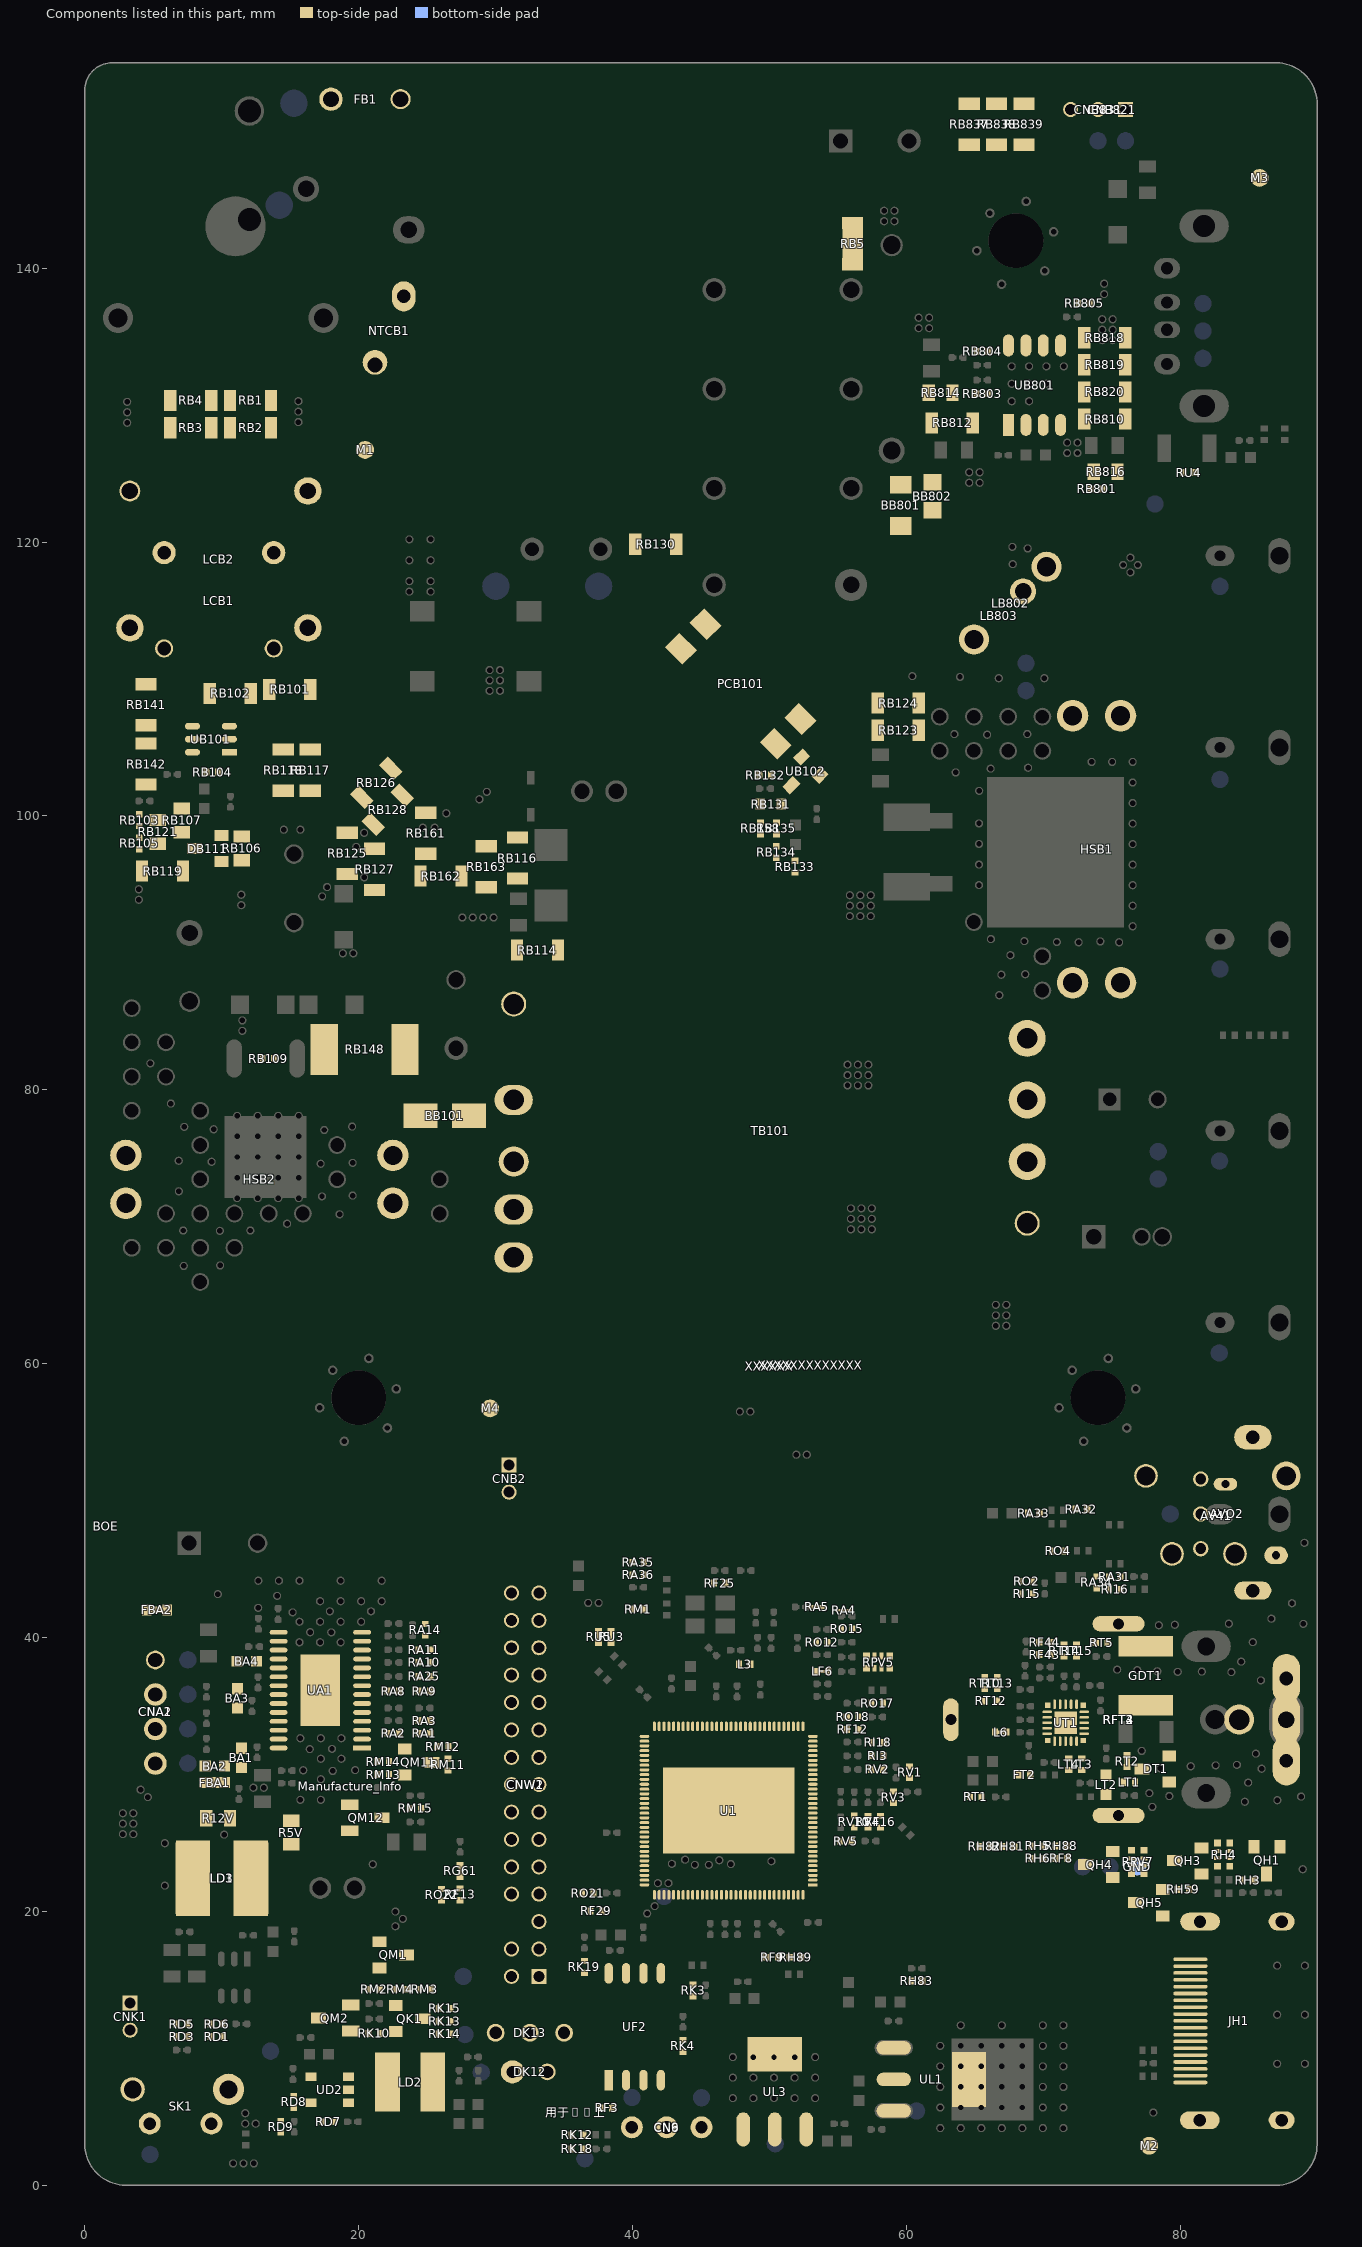
[diagram p0: the components of this part, seen from the top]
# Altium PCB MISC116569.PcbDoc (part 4 of 15)
Units mm, origin at the board's own origin, x right, y up, seen from the top; angles counter-clockwise.
Board outline 90 x 155 mm, 2 copper layers (TopLayer, BottomLayer), stack 1.571 mm thick; 527 components, 277 nets, 2450 pads, 649 vias.

## Footprints (in the part's own frame and the unit in brackets; to place one, negate y for a bottom-side part, rotate by r counter-clockwise, add the part's x,y. Pads: shape width x height; smd on the part's side, far side on the other; paste and mask are expansions set on the pad) (continued)
"FUSE8.5*4-V-5(T3.15AL 250V~)" [mm] "SMT1315AP/2010T1A250VA1(编带/华德)"
  round 1.7 hole 1.15: 1(2.54,0)
  round 1.473 / inner round 1.7 / far side round 1.7 hole 1.15: 2(-2.54,0)
  round 1.9 on Top Overlay: 4(2.54,0) 5(-2.54,0)
  BottomLayer lines w1: 2.54,0 2.562,-0.022 3.977,-1.437 ; 2.312,-0.271 2.338,-0.289 2.367,-0.31 3.499,-1.103 3.977,-1.437 ; -2.312,0.271 -2.338,0.289 -2.376,0.316 -2.933,0.706 -3.977,1.437 ; -2.54,0 -3.011,0.471 -3.977,1.437 ; -2.811,-0.228 -2.829,-0.202 ; 3.977,-1.437 2.971,0 2.844,0.182 ; 2.844,0.182 2.844,0.182 ; 2.844,0.182 2.829,0.202 2.812,0.227 ; 2.812,0.227 2.811,0.228 ; -2.829,-0.202 -2.839,-0.189 -2.973,0.003 -3.096,0.179 -3.165,0.277 -3.828,1.224 -3.977,1.437 ; -2.829,-0.202 -2.829,-0.202 ; -2.829,-0.202 -2.829,-0.202 ; -3.977,1.437 -3.977,1.437
  silkscreen extent -4.3,-2.1 4.3,2.1, body extent -4.3,-2.1 4.3,2.1, height 8.5
GND#1 [mm] "导通线"
  rect 0.66x0.178 smd paste-0.45 mask-0.45: JP_1K(-0.32,0) JP_2K(0.32,0)
GND#2 [mm] "导通线"
  rect 0.66x0.3 smd paste-0.45 mask-0.45: JP_1K(-0.32,0) JP_2K(0.32,0)
HDMI-HS-1 [mm] "浙江和丰   HHF-14B000-2SA。17.09.25更新钢网;171107更新焊盘露铜位置;18.04.19 更新大脚孔径;19.09.11 更新端子视图开口高度(6.1-6.2,0."
  rect 2.2x3.8 on Top Paste: 0(-7.75,4.18) 0(7.753,4.183)
  rect 2.2x6 on Top Paste: 0(-7.75,9.355) 0(7.75,9.355)
  oval 0.26x2.5 smd: 1(4.5,11.258) 2(4,11.258) 3(3.5,11.258) 4(3,11.258) 5(2.5,11.258) 6(2,11.258) 7(1.5,11.258) 8(1,11.258) 9(0.5,11.258) 10(0,11.258) 11(-0.5,11.258) 12(-1,11.258) 13(-1.5,11.258) 14(-2,11.258) 15(-2.5,11.258) 16(-3,11.258) 17(-3.5,11.258) 18(-4,11.258) 19(-4.5,11.258)
  oval 1.3x2.9 hole 0.9 slot 2.5 at 90 deg mask+0.076: 20(-7.25,10.565) 22(7.25,10.55)
  oval 1.3x1.9 hole 0.9 slot 1.5 at 90 deg mask+0.076: 21(-7.25,4.59) 23(7.25,4.59)
  silkscreen extent -7.5,2 7.5,12.19, body extent -10.25,-57.68 10.25,12.17, height 8.92
"Heat-Shrinkable Tube" [mm] "收缩前壁厚0.3+-0.05，收缩后壁厚0.6+-0.1"
  round 0.3 on Mech2: 0(0,0)
"High Voltage" [mm]
  silkscreen extent -0.53,-1.52 0.43,1.27
HOT [mm]
HS151-TEMP-NG [mm] "散热片.临时封装.10/21/2019"
  oval 1.9x2.4 on Top Overlay: 0(-9.75,-1.75) 0(-9.75,1.75) 0(9.75,-1.75) 0(9.75,1.75)
  round 3 on Bottom Solder: 0(-9.75,-1.75) 0(-9.75,1.75) 0(9.75,-1.75) 0(9.75,1.75)
  round 2.3 hole 1.4: 1(-9.75,1.75) 2(-9.75,-1.75) 3(9.75,-1.75) 4(9.75,1.75)
  silkscreen extent -10.03,-2.93 10.03,2.93
HS(15X15X5)-S [mm] "YT.YT-P-151505.2019/9/18"
  silkscreen extent -7.63,-7.63 7.63,7.63, body extent -7.5,-7.5 7.5,7.5, height 5
KEY-HD-6 [mm] "春生KFC-A06--E-4-160-7.5/4; 中心高度为4mm;14.09.04;171102修正突出距离"
  round 2.5 on Top Overlay: 0(-3.5,5) 0(3.5,5)
  round 1.8 on Top Overlay: 0(-2.25,2.5) 0(2.25,2.5)
  round 1.6 hole 0.9: 1(2.25,2.5) 2(-2.25,2.5)
  round 2.286 hole 1.3: 3(3.5,5)
  round 1.778 / inner round 2.286 / far side round 2.286 hole 1.3: 4(-3.5,5)
  silkscreen extent -3.85,0 3.85,6.6
L0402 [mm] "电感"
  rect 0.45x0.55 smd mask+0.076: 1(-0.425,0) 2(0.425,0)
  silkscreen extent -0.8,-0.42 0.8,0.43, body extent -0.5,-0.25 0.5,0.25, height 0.5
L0603 [mm] "片式磁珠、电感、ESD"
  rect 0.813x0.8 smd mask+0.076: 1(-0.706,0) 2(0.706,0)
  silkscreen extent -1.27,-0.55 1.27,0.55, body extent -0.8,-0.4 0.8,0.4, height 0.8
L0805 [mm] "片式磁珠、电感"
  rect 1.2x1.3 smd: 1(-1.016,0) 2(1.016,0)
  silkscreen extent -1.92,-0.95 1.92,0.95, body extent -1,-0.62 1,0.63, height 1.25
L1206 [mm] "磁珠"
  rect 1.3x1.6 smd: 1(-1.5,-0.001) 2(1.5,0.001)
  silkscreen extent -2.55,-1.2 2.55,1.2, body extent -1.6,-0.8 1.6,0.8, height 1.25
L(4*3*2.55)-S [mm] "贴片磁珠；SMB -302540-K5B- L1;15.02.05（17.12.07更新高度信息）"
  rect 2.5x1.8 smd: 1(-1.775,0) 2(1.775,0)
  silkscreen extent -2.12,-1.6 2.12,1.6, body extent -2.55,-1.6 2.55,1.6, height 2.7
L(4.5*3.5)-S [mm] "SMD4532-6R8M-023"
  rect 1.8x4.3 smd: 1(-1.65,0) 2(1.65,0)
  TopLayer pour cut-out: -0.76,2.15 0.796,2.15 0.796,2.141 0.796,-2.149 -0.756,-2.149 -0.756,-2.15
  silkscreen extent -2.83,-2.44 3.3,2.44
L(5.8*4.5)-S [mm] "APC52A45M4R7\电感\Cailank;170317更新阻焊兼容L(4*3.0)-S"
  rect 2.5x5.5 smd paste-5.5: 1(2.105,0) 2(-2.105,0)
  TopLayer pour cut-out: -0.849,2.746 -0.845,2.75 0.861,2.75 0.861,-2.749 0.861,-2.753 0.859,-2.753 -0.862,-2.753
  silkscreen extent -1.5,-2.9 3.88,2.9, body extent -3.06,-2.65 3.08,2.74, height 4.8
L(6.0*4.5)-S [mm] "SWPA6045S4R7MT(Sunlord) :功率电感;161103更新焊盘大小"
  rect 2.1x5.2 smd paste-6: 1(-2.35,0) 2(2.35,0)
  TopLayer pour cut-out: -1.282,2.552 1.294,2.543 1.297,-2.547 -1.311,-2.549
  silkscreen extent -3.16,-3.15 3.9,3.15, body extent -3,-3 3,3, height 4.5
L(13.5*15.5)-V-5 [mm] "深圳秀益达；SA-A048-036-A SPK1214RBL-680K；14.11.19"
  round 1.9 hole 1.2 mask+0.076: 1(-2.5,0) 2(2.5,0)
  round 2.1 on Top Overlay mask+0.076: 3(-2.5,0) 4(2.5,0)
  silkscreen extent -6.75,-6.75 6.75,6.75, body extent -9.53,-9.51 9.52,9.53, height 15.5
L/LC2/15*14.5-V7.5 [mm] "SYDR1212-L003-YMX"
  round 2.2 hole 1.4: 1(-3.75,0) 2(3.75,0)
  round 2.4 on Top Overlay: 1(-3.75,0) 1(3.75,0)
  silkscreen extent -7.25,-7.25 7.25,7.25
L/LC4/UU9.8/7*8-H [mm] "汉(玛电子UU9.8-26mH)"
  round 1.7 hole 1: 1(-4,-3.5) 2(4,-3.5)
  round 1.321 / inner round 1.7 / far side round 1.7 hole 1: 3(4,3.5) 4(-4,3.5)
  round 1.9 on Top Overlay: 17(-4,3.5) 18(4,3.5) 19(4,-3.5) 20(-4,-3.5)
  silkscreen extent -8.5,-11 8.5,5
L/UU10.5/10*13-2 [mm] "SYUU10.5-L001(协兴电子) 卡扣在侧面"
  round 2 hole 1.2: 1(5,-6.5) 3(-5,6.5) 4(-5,-6.5)
  round 1.524 / inner round 2 / far side round 2 hole 1.2: 2(5,6.5)
  round 2.2 on Top Overlay: 4(-5,6.5) 4(-5,-6.5) 4(5,6.5) 4(5,-6.5)
  silkscreen extent -8,-9.25 11.5,9.25, body extent -8,-8.5 9.5,8.5, height 13.8
LED-HD-5 [mm] "HZFT503094CPBR-1(红、蓝);14.06.27"
  oval 1.5x1.7 on Top Overlay: 0(-2.502,0.002) 0(-0.002,0.002) 0(2.498,0.002)
  round 1.3 / inner oval 1.3x1.5 / far side oval 1.5x2 hole 0.9: 1(-2.502,0.002) 2(-0.002,0.002) 3(2.498,0.002)
  silkscreen extent -2.81,-11.06 2.8,2.6
LED-HD-6 [mm] "厦门华联；HFR803099P(P5D2)-S5(SN)；14.09.03"
  round 1.9 on Top Overlay mask+0.076: 3(1.27,2.65) 4(-1.27,2.65)
  round 1.7 hole 0.9 mask+0.076: A(-1.27,2.65)
  round 1.219 / inner round 1.7 / far side round 1.7 hole 0.9 mask+0.076: K(1.27,2.65)
  silkscreen extent -2.02,-5.62 2.02,4.02
MANUFACTURE_INFO [mm]
  round 0.3 on Mech2: 0(0,0)
MARK [mm] "SMD 使用"
  round 1.3 smd paste+0 mask+0.65: 0(0,0)
  TopLayer circle w0.254: c0,0 r1.444
  TopLayer pour cut-out: -1.3,0 -1.201,-0.497 -0.919,-0.919 -0.497,-1.201 0,-1.3 0,-1.3 0.497,-1.201 0.919,-0.919 1.201,-0.497 1.3,0 1.3,0 1.201,0.497 0.919,0.919 0.497,1.201 0,1.3 0,1.3 -0.497,1.201 -0.919,0.919 -1.201,0.497 -1.3,0
Mylar [mm] "180×180×0.4mm-PC-黑色"
NTC(10*5)-V5 [mm] "热敏电阻 SCK152R58MSY  (为勤电子）;161022更新椭圆孔"
  round 1.8 hole 1.1 copper offset 0.178,0: 1(-2.5,1.05)
  round 2 on Top Overlay: 2(-2.5,1.05)
  oval 2.2x1.7 hole 1 slot 1.5 at 0 deg: 2(2.5,-1.05)
  oval 2.4x1.9 on Top Overlay: 3(2.5,-1.05)
  silkscreen extent -5.77,-2.5 5.77,2.5, body extent -5.75,-2 5.75,2, height 13.75
OC4-S-1 [mm] "巨路国际；肖特基LTV-817S-TA-B"
  rect 1.5x1.8 smd: 1(-1.27,-4.9) 2(1.27,-4.9) 3(1.27,4.9) 4(-1.27,4.9)
  silkscreen extent -3.17,-5.35 2.55,3.5, body extent -6.95,-6.95 6.95,6.95, height 3.88
OPTICAL-HD-3 [mm] "强生GQ-03-08  通用封装 (TR）  塑胶整体高度11.6mm，中心高度6mm(17.04.28,增加丝印宽度到12.3mm）"
  oval 2x3.4 on Top Overlay: 0(-5.6,4.7) 0(5.6,4.7)
  round 1.778 on Top Overlay: 0(-2.54,8.5) 0(0,8.5) 0(2.54,8.5)
  round 1.118 / inner round 1.524 / far side round 1.524 hole 0.8: 1(-2.54,8.5) 2(0,8.5) 3(2.54,8.5)
  oval 1.321x2.718 / inner oval 1.8x3.2 / far side oval 1.8x3.2 hole 1 slot 2.4 at 90 deg: 4(-5.6,4.7)
  oval 1.8x2.718 / inner oval 1.8x3.2 / far side oval 1.8x3.2 hole 1 slot 2.4 at 90 deg: 5(5.6,4.7)
  silkscreen extent -6.15,0 6.15,11.8
PCB_NAME [mm]
  round 0.3 on Mech2: 0(0,0)
PCB_TIME [mm]
  round 0.3 on Mech2: 0(0,0)
PHONE-HD-42 [mm] "YUQIU;PJ7724-F05L3BE-D;160401(17.07.18,孔内边增加0.1mm，外距不变）(18.03.13 更新孔径）"
  oval 1.5x2.3 on Top Overlay: 0(-3,3) 8(2.2,6.7)
  round 2.3 on Top Overlay: 0(-2.9,10.6) 0(-2.9,6) 0(2.8,12.5) 0(2.8,2.25)
  round 2.1 hole 1.4: 1(2.8,2.25)
  oval 1.3x1.727 / inner oval 1.3x2.1 / far side oval 1.3x2.1 hole 0.6 slot 1.4 at 90 deg: 2(-3,3)
  round 1.727 / inner round 2.1 / far side round 2.1 hole 1.4: 3(2.8,12.5) 4(-2.9,6) 5(-2.9,10.6)
  oval 0.914x1.727 / inner oval 1.3x2.1 / far side oval 1.3x2.1 hole 0.6 slot 1.4 at 90 deg: 6(2.2,6.7)
  silkscreen extent -3.65,0 3.65,13.15, body extent -5.05,-62.22 5.05,13, height 12.05
QFN24/0.4-1 [mm] "Si2151;14-03-17;161116新增两个EPAD孔"
  rect 0.4x0.4 smd: 1(-1.295,1.295) 7(-1.295,-1.295) 13(1.295,-1.295) 19(1.295,1.295)
  oval 0.7x0.2 smd: 2(-1.35,0.8) 3(-1.35,0.4) 4(-1.35,0) 6(-1.35,-0.8) 14(1.35,-0.8) 15(1.35,-0.4) 16(1.35,0) 17(1.35,0.4) 18(1.35,0.8)
  oval 0.7x0.2 smd paste+0: 5(-1.35,-0.4)
  oval 0.2x0.7 smd: 8(-0.8,-1.35) 9(-0.4,-1.35) 10(0,-1.35) 11(0.4,-1.35) 12(0.8,-1.35) 20(0.8,1.35) 21(0.4,1.35) 22(0,1.35) 23(-0.4,1.35)
  oval 0.2x0.7 smd paste+0: 24(-0.8,1.35)
  rect 1.651x1.651 smd paste-2 mask-2: EPAD(0,0)
  silkscreen extent -2.6,-2.24 2.11,2.24, body extent -1.5,-1.5 1.5,1.5, height 0.9
QFN128/0.35-1 [mm] "Mstar,TSUMV53RWUT-Z1,18.11.16(19.03.30   减少外延焊盘长度）(19.04.23 更新钢网尺寸）（因温升修改为12宫格）"
  oct 2.2x1.9 on Top Paste: 0(-3.7,0) 0(-3.697,-2.145) 0(-3.697,2.145) 0(-1.253,2.145) 0(-1.253,-2.145) 0(-1.25,0) 0(1.247,2.145) 0(1.247,-2.145) 0(1.25,0) 0(3.697,-2.145) 0(3.697,2.145) 0(3.7,0)
  oct 2.2x1.9 on Top Solder: 0(-3.7,0) 0(-3.697,-2.145) 0(-3.697,2.145) 0(-1.253,2.145) 0(-1.253,-2.145) 0(-1.25,0) 0(1.247,2.145) 0(1.247,-2.145) 0(1.25,0) 0(3.697,-2.145) 0(3.697,2.145) 0(3.7,0)
  rect 0.7x0.22 smd paste-0.02 mask-0.035: 1(-6.151,5.425)
  oval 0.7x0.22 smd paste-0.02 mask-0.035: 2(-6.151,5.075) 3(-6.151,4.725) 4(-6.151,4.375) 5(-6.151,4.025) 6(-6.151,3.675) 7(-6.151,3.325) 8(-6.151,2.975) 9(-6.151,2.625) 10(-6.151,2.275) 11(-6.151,1.925) 12(-6.151,1.575) 13(-6.151,1.225) 14(-6.151,0.875) 15(-6.151,0.525) 16(-6.151,0.175) 17(-6.151,-0.175) 18(-6.151,-0.525) 19(-6.151,-0.875) 20(-6.151,-1.225) 21(-6.151,-1.575) 22(-6.151,-1.925) 23(-6.151,-2.275) 24(-6.151,-2.625) 25(-6.151,-2.975) 26(-6.151,-3.325) 27(-6.151,-3.675) 28(-6.151,-4.025) 29(-6.151,-4.375) 30(-6.151,-4.725) 31(-6.151,-5.075) 32(-6.151,-5.425) 65(6.151,-5.425) 66(6.151,-5.075) 67(6.151,-4.725) 68(6.151,-4.375) 69(6.151,-4.025) 70(6.151,-3.675) 71(6.151,-3.325) 72(6.151,-2.975) 73(6.151,-2.625) 74(6.151,-2.275) 75(6.151,-1.925) 76(6.151,-1.575) 77(6.151,-1.225) 78(6.151,-0.875) 79(6.151,-0.525) 80(6.151,-0.175) 81(6.151,0.175) 82(6.151,0.525) 83(6.151,0.875) 84(6.151,1.225) 85(6.151,1.575) 86(6.151,1.925) 87(6.151,2.275) 88(6.151,2.625) 89(6.151,2.975) 90(6.151,3.325) 91(6.151,3.675) 92(6.151,4.025) 93(6.151,4.375) 94(6.151,4.725) 95(6.151,5.075) 96(6.151,5.425)
  oval 0.22x0.7 smd paste-0.02 mask-0.035: 33(-5.425,-6.151) 34(-5.075,-6.151) 35(-4.725,-6.151) 36(-4.375,-6.151) 37(-4.025,-6.151) 38(-3.675,-6.151) 39(-3.325,-6.151) 40(-2.975,-6.151) 41(-2.625,-6.151) 42(-2.275,-6.151) 43(-1.925,-6.151) 44(-1.575,-6.151) 45(-1.225,-6.151) 46(-0.875,-6.151) 47(-0.525,-6.151) 48(-0.175,-6.151) 49(0.175,-6.151) 50(0.525,-6.151) 51(0.875,-6.151) 52(1.225,-6.151) 53(1.575,-6.151) 54(1.925,-6.151) 55(2.275,-6.151) 56(2.625,-6.151) 57(2.975,-6.151) 58(3.325,-6.151) 59(3.675,-6.151) 60(4.025,-6.151) 61(4.375,-6.151) 62(4.725,-6.151) 63(5.075,-6.151) 64(5.425,-6.151) 97(5.425,6.151) 98(5.075,6.151) 99(4.725,6.151) 100(4.375,6.151) 101(4.025,6.151) 102(3.675,6.151) 103(3.325,6.151) 104(2.975,6.151) 105(2.625,6.151) 106(2.275,6.151) 107(1.925,6.151) 108(1.575,6.151) 109(1.225,6.151) 110(0.875,6.151) 111(0.525,6.151) 112(0.175,6.151) 113(-0.175,6.151) 114(-0.525,6.151) 115(-0.875,6.151) 116(-1.225,6.151) 117(-1.575,6.151) 118(-1.925,6.151) 119(-2.275,6.151) 120(-2.625,6.151) 121(-2.975,6.151) 122(-3.325,6.151) 123(-3.675,6.151) 124(-4.025,6.151) 125(-4.375,6.151) 126(-4.725,6.151) 127(-5.075,6.151) 128(-5.425,6.151)
  rect 9.6x6.3 smd paste-6 mask-6: EPAD(0,0)
  silkscreen extent -7.48,-7.42 7.42,7.4, body extent -6.2,-6.2 6.2,6.2, height 0.95
R0402 [mm] "片式电阻"
  rect 0.45x0.5 smd mask+0.076: 1(-0.425,0) 2(0.425,0)
  silkscreen extent -0.8,-0.4 0.8,0.4, body extent -0.5,-0.25 0.5,0.25, height 0.5
R0402SC#1 [mm]
  rect 0.45x0.5 smd mask+0.076: 1(-0.425,0) 2(0.425,0)
  rect 0.42x0.25 smd paste-0.5 mask-0.5: 3(0,0)
  silkscreen extent -0.8,-0.4 0.8,0.4, body extent -0.5,-0.25 0.5,0.25, height 0.5
R0402SC#2 [mm]
  rect 0.45x0.5 smd mask+0.076: 1(-0.425,0) 2(0.425,0)
  rect 0.42x0.401 smd paste-0.5 mask-0.5: 3(0,0)
  silkscreen extent -0.8,-0.4 0.8,0.4, body extent -0.5,-0.25 0.5,0.25, height 0.5
R0603 [mm] "贴片电阻"
  rect 0.7x0.8 smd mask+0.076: 1(-0.756,0) 2(0.756,0)
  silkscreen extent -1.25,-0.54 1.25,0.54, body extent -0.8,-0.4 0.8,0.4, height 0.8
R0603SC#1 [mm] "贴片电阻"
  rect 0.7x0.8 smd mask+0.076: 1(-0.756,0) 2(0.756,0)
  rect 0.82x0.813 smd paste-0.5 mask-0.5: 3(0,0)
  silkscreen extent -1.25,-0.54 1.25,0.54, body extent -0.8,-0.4 0.8,0.4, height 0.8
R0603SC#2 [mm] "贴片电阻"
  rect 0.7x0.8 smd mask+0.076: 1(-0.756,0) 2(0.756,0)
  rect 0.82x0.5 smd paste-0.5 mask-0.5: 3(0,0)
  silkscreen extent -1.25,-0.54 1.25,0.54, body extent -0.8,-0.4 0.8,0.4, height 0.8
R0805 [mm] "贴片电阻"
  rect 0.9x1.2 smd mask+0.076: 1(-0.866,0) 2(0.866,0)
  silkscreen extent -1.47,-0.75 1.47,0.75, body extent -1,-0.62 1,0.63, height 0.5
R1206 [mm] "贴片电阻"
  rect 0.9x1.55 smd mask+0.076: 1(-1.5,0) 2(1.5,0)
  silkscreen extent -2.1,-0.93 2.1,0.93, body extent -1.6,-0.8 1.6,0.8, height 0.55
R1206SC [mm] "贴片电阻"
  rect 0.9x1.55 smd mask+0.076: 1(-1.5,0) 2(1.5,0)
  rect 2.7x1.5 smd paste-2.7 mask-2.7: 3(0,0)
  silkscreen extent -2.1,-0.93 2.1,0.93, body extent -1.6,-0.8 1.6,0.8, height 0.55
R2512-1 [mm] "PSA;Size 2512 2W;16.01.20(17.06.19修改焊盘大小，增强爬锡，解决浮高问题）"
  rect 2x3.7 smd: 1(-2.95,0) 2(2.95,0)
  silkscreen extent -3.3,-2 3.3,2, body extent -3.25,-1.65 3.25,1.65, height 0.75
RA0402 [mm] "排阻"
  rect 0.5x0.5 smd mask+0.076: 1(-0.45,0.85) 2(0.45,0.85) 7(-0.45,-0.85) 8(0.45,-0.85)
  rect 0.5x0.3 smd mask+0.076: 3(-0.45,0.25) 4(0.45,0.25) 5(-0.45,-0.25) 6(0.45,-0.25)
  silkscreen extent -0.85,-1.27 0.85,1.27, body extent -0.51,-1 0.51,1, height 0.35
REMOTE-VD-6 [mm] "ALL-BEST,ARM-383AW1-Z-R-D10-22,18.11.21"
  round 1.8 on Top Overlay: 0(-2.54,2) 0(0,2) 0(2.54,2)
  round 1.6 hole 0.9: 1(-2.54,2) 2(0,2) 3(2.54,2)
  silkscreen extent -3.1,-2 3.1,3.4
REMOTE-VD-9 [mm] "Fantasy.FDI-M6069560R538-WJGC25-D22.2019/8/23"
  round 1.7 on Top Overlay: 0(-2.54,0.05) 0(0,0) 0(2.54,0.05)
  round 1.5 hole 0.9: 1(-2.54,0.05) 2(0,0) 3(2.54,0.05)
  silkscreen extent -3.15,-4.2 3.15,1.7
SFQ [mm]
  silkscreen extent 0,-0.72 2.37,0.72
"Silica gel-5*3" [mm] "硅胶5*3mm,用于插件IR或者同轴光纤座子点胶,1013_2018"
  silkscreen extent -1.5,-2.5 1.5,2.5
"Silica gel-10" [mm] "硅胶"
  silkscreen extent -3,-5 3,5
"Silica gel-15" [mm] "硅胶"
  silkscreen extent -3,-7.5 3,7.5
SIP2*15/2.0D-2 [mm] "捷仕泰-XXXXXXXXXXX 12106专用，缺第六脚/LK-HEPHM20012150-006"
  round 1.3 on Top Overlay: 0(-14,-1) 0(-14,1) 0(-12,-1) 0(-12,1) 0(-10,-1) 0(-10,1) 0(-8,-1) 0(-8,1) 0(-6,-1) 0(-6,1) 0(-4,-1) 0(-4,1) 0(-2,-1) 0(-2,1) 0(0,-1) 0(0,1) 0(2,-1) 0(2,1) 0(4,-1) 0(4,1) 0(6,-1) 0(6,1) 0(8,-1) 0(8,1) 0(10,1) 0(12,-1) 0(12,1) 0(14,-1)
  round 1.3 on Bottom Solder: 0(10,-1)
  rect 1.3x1.3 on Top Overlay: 0(14,1)
  rect 1.1x1.1 hole 0.8: 1(14,1)
  round 1.1 hole 0.8: 2(14,-1) 3(12,1) 4(12,-1) 5(10,1) 7(8,1) 8(8,-1) 9(6,1) 10(6,-1) 11(4,1) 12(4,-1) 13(2,1) 14(2,-1) 15(0,1) 16(0,-1) 17(-2,1) 18(-2,-1) 19(-4,1) 20(-4,-1) 21(-6,1) 22(-6,-1) 23(-8,1) 24(-8,-1) 25(-10,1) 26(-10,-1) 27(-12,1) 28(-12,-1) 29(-14,1) 30(-14,-1)
  silkscreen extent -15.1,-3 15.65,3, body extent -15,-2.1 15,2.1, height 6
SIP2*15/2.0D-11 [mm] "浙江创佳；PHD-2*n-DK-6;,缺第6PIN；14.12.04"
  round 1.3 on Bottom Solder: 0(10,-1)
  rect 1.1x1.1 hole 0.8: 1(14,1)
  round 1.1 hole 0.8: 2(14,-1) 3(12,1) 4(12,-1) 5(10,1) 7(8,1) 8(8,-1) 9(6,1) 10(6,-1) 11(4,1) 12(4,-1) 13(2,1) 14(2,-1) 15(0,1) 16(0,-1) 17(-2,1) 18(-2,-1) 19(-4,1) 20(-4,-1) 21(-6,1) 22(-6,-1) 23(-8,1) 24(-8,-1) 25(-10,1) 26(-10,-1) 27(-12,1) 28(-12,-1) 29(-14,1) 30(-14,-1)
  rect 1.3x1.3 on Top Overlay: 372(14,1)
  round 1.3 on Top Overlay: 373(12,1) 374(-10,-1) 374(10,1) 375(8,1) 376(6,1) 377(4,1) 378(2,1) 379(0,1) 380(-2,1) 381(-4,1) 382(-6,1) 383(-8,1) 384(-10,1) 385(-12,1) 386(-14,1) 387(14,-1) 388(12,-1) 390(8,-1) 391(6,-1) 392(4,-1) 393(2,-1) 394(0,-1) 395(-2,-1) 396(-4,-1) 397(-6,-1) 398(-8,-1) 400(-12,-1) 401(-14,-1)
  silkscreen extent -16.12,-3.47 16.59,3.53, body extent -16.03,-2.5 16,3.25, height 6.5
SIP2/2.0D-1 [mm] "捷仕泰/铭锋达"
  rect 1.3x1.3 on Top Overlay: 0(-1,0)
  round 1.3 on Top Overlay: 0(1,0)
  rect 1.1x1.1 hole 0.8: 1(-1,0)
  round 1.1 hole 0.8: 2(1,0)
  silkscreen extent -3,-3.2 3,1.8, body extent -3,-3.2 3,1.8, height 6
SIP3/2.0D-3 [mm] "捷仕泰   A2004-03-A1MA-P,插线高度11mm"
  rect 1.5x1.5 on Top Overlay: 0(-2,0)
  round 1.5 on Top Overlay: 0(0,0) 0(2,0)
  rect 1.1x1.1 hole 0.8: 1(-2,0)
  round 1.1 hole 0.8: 2(0,0) 3(2,0)
  silkscreen extent -4,-2.13 4,3.07, body extent -4,-2.18 4,3.1, height 7.8
SIP4/2.5D-2 [mm]
  rect 1.905x1.905 on Top Overlay: 0(-3.78,0)
  round 1.905 on Top Overlay: 0(-1.26,0) 0(1.26,0) 0(3.78,0)
  round 1.372 / inner round 1.651 / far side rect 1.651x1.651 hole 1.05: 1(-3.78,0)
  round 1.651 hole 1.05: 2(-1.26,0) 3(1.26,0) 4(3.78,0)
  silkscreen extent -6.4,-3.6 6.4,3
SIP4/2.54D-1 [mm] "捷仕泰/铭锋达"
  rect 1.905x1.905 on Top Overlay: 0(-3.78,0)
  round 1.905 on Top Overlay: 0(-1.26,0) 0(1.26,0) 0(3.78,0)
  round 1.372 / inner round 1.651 / far side rect 1.651x1.651 hole 1.05: 1(-3.78,0)
  round 1.651 hole 1.05: 2(-1.26,0) 3(1.26,0) 4(3.78,0)
  silkscreen extent -6.44,-3.5 6.44,2.5, body extent -6.35,-3.5 6.35,2.5, height 7
SMD4532-1 [mm] "Brightking,4532-091-LF,气体放电管,雷电防护器件，17.06.12"
  rect 1.5x4 smd: 1(-2.15,0) 2(2.151,0)
  silkscreen extent -1.25,-1.79 1.23,1.71, body extent -2.41,-1.75 2.41,1.75, height 3
SO-8A [mm] "FLASH"
  rect 1.6x0.8 smd: 1(-2.9,1.905)
  oval 1.6x0.8 smd: 2(-2.9,0.635) 3(-2.9,-0.635) 4(-2.9,-1.905) 5(2.9,-1.905) 6(2.9,-0.635) 7(2.9,0.635) 8(2.9,1.905)
  silkscreen extent -4.71,-2.54 2,2.54, body extent -3.1,-2.5 3.1,2.5, height 1.76
SO-23 [mm] "双向二极管封装"
  rect 0.8x1 smd: 1(0.952,1.016) 3(-0.953,1.016)
  rect 0.8x1.1 smd: 2(0,-0.966)
  silkscreen extent -1.55,-0.86 1.55,0.36, body extent -1.5,-1.25 1.5,1.25, height 1.1
SOIC8 [mm] "W25X40BVSNIG/GD25Q32BSIG/GD25LQ16"
  rect 1.5x0.6 smd: 1(-3.9,1.905)
  oval 1.5x0.6 smd: 2(-3.9,0.635) 3(-3.9,-0.635) 4(-3.9,-1.905) 5(3.9,-1.905) 6(3.9,-0.635) 7(3.9,0.635) 8(3.9,1.905)
  silkscreen extent -4.28,-2.65 2.7,3.53, body extent -4.05,-2.69 4.05,2.69, height 2.17
SOP28/0.65-7 [mm] "ESMT,AD52050B-26QG28NRR,0723_2018"
  oct 1.2x1 on Top Paste mask+0: 0(-0.75,1.95) 0(-0.75,0.65) 0(-0.75,-0.65) 0(-0.75,-1.95) 0(0.75,1.95) 0(0.75,0.65) 0(0.75,-0.65) 0(0.75,-1.95)
  oct 1.2x1 on Top Solder mask+0: 0(-0.75,1.95) 0(-0.75,0.65) 0(-0.75,-0.65) 0(-0.75,-1.95) 0(0.75,1.95) 0(0.75,0.65) 0(0.75,-0.65) 0(0.75,-1.95)
  rect 1.3x0.35 smd mask+0.051: 1(-3.05,4.225)
  oval 1.3x0.35 smd mask+0.051: 2(-3.05,3.575) 3(-3.05,2.925) 4(-3.05,2.275) 5(-3.05,1.625) 6(-3.05,0.975) 7(-3.05,0.325) 8(-3.05,-0.325) 9(-3.05,-0.975) 10(-3.05,-1.625) 11(-3.05,-2.275) 12(-3.05,-2.925) 13(-3.05,-3.575) 14(-3.05,-4.225) 15(3.05,-4.225) 16(3.05,-3.575) 17(3.05,-2.925) 18(3.05,-2.275) 19(3.05,-1.625) 20(3.05,-0.975) 21(3.05,-0.325) 22(3.05,0.325) 23(3.05,0.975) 24(3.05,1.625) 25(3.05,2.275) 26(3.05,2.925) 27(3.05,3.575) 28(3.05,4.225)
  rect 2.9x5.2 smd paste-5 mask-5: EPAD(0,0)
  silkscreen extent -4.95,-4.9 4.44,4.9, body extent -3.2,-4.9 3.2,4.9, height 1.2
SOT-23 [mm]
  rect 0.8x1 smd: B(0.953,1.016) E(-0.953,1.016)
  rect 0.8x1.1 smd: C(-0.013,-0.966)
  silkscreen extent -1.55,-0.81 1.55,0.36, body extent -1.5,-1.25 1.5,1.25, height 1.1
SOT-23-1 [mm]
  rect 0.8x1.1 smd: D(0,-1.15)
  rect 0.8x1.27 smd: G(0.95,1.2) S(-0.95,1.2)
  TopLayer pour cut-out: -1.583,0.903 -1.583,-0.905 1.587,-0.905 1.587,0.903
  silkscreen extent -1.55,-1.05 1.55,0.33, body extent -1.52,-1.48 1.52,1.48, height 1.25
SOT-23-5 [mm] "LPW5206(1.295mm)"
  rect 0.6x0.8 smd: 1(-0.95,-1.375) 2(0,-1.375) 3(0.95,-1.375) 4(0.95,1.375) 5(-0.95,1.375)
  silkscreen extent -1.5,-2.49 1.5,0.85, body extent -1.5,-0.85 1.5,0.85, height 1.45
SOT-23-RAK [mm] "TL431G-AE2-R(UTC)"
  rect 0.8x1.1 smd: A(0.013,0.966)
  rect 0.8x1 smd: K(0.952,-1.016) R(-0.953,-1.016)
  silkscreen extent -1.52,-0.36 1.52,0.86, body extent -1.5,-1.25 1.5,1.25, height 1.1
SOT-26 [mm] "LD7536R"
  rect 0.5x1.1 smd: 1(0.95,1.35)
  oval 0.5x1.1 smd: 2(0,1.35) 3(-0.95,1.35) 4(-0.95,-1.35) 5(0,-1.35) 6(0.95,-1.35)
  silkscreen extent -1.55,-2.54 1.55,2.9, body extent -1.55,-0.9 1.55,0.9, height 1.45
SOT-223 [mm]
  oval 1x2.5 smd: 1(-2.3,-2.75) 2(0,-2.75) 3(2.3,-2.75)
  rect 4x2.5 smd: 4(0,2.75)
  TopLayer pour cut-out: 2.3,-1.188 2.3,-4.312 -2.345,-4.312 -2.64,-4.253 -2.891,-4.086 -3.058,-3.835 -3.117,-3.54 -3.117,-3.54 -2.299,-3.54 -2.299,-1.956 -3.124,-1.956 -3.066,-1.662 -2.899,-1.413 -2.65,-1.247 -2.356,-1.188 -2.356,-1.188
  silkscreen extent -3.45,-2.75 3.45,2.81, body extent -3.35,-3.3 3.35,3.4, height 1.7
T-14.5×25×9.0-IEC14.5 [mm] "14.5×25×9.0-IEC14.5 中心出口高度6.3mm (已开模）"
  oval 2.1x4.1 on Top Overlay: 1(-7,12.25)
  oval 4.1x2.1 on Top Overlay: 1(0,24.5)
  round 2.1 hole 1.3: 1(0,3.45)
  oval 3.8x2.1 on Top Overlay: 1(0,0)
  oval 1.778x4.1 on Top Overlay: 1(7,12.25)
  oval 3.6x2 hole 1 slot 2.6 at 0 deg: 2(0,0)
  oval 1.118x3.8 / inner oval 1.8x3.8 / far side oval 1.8x3.8 hole 0.8 slot 2.8 at 90 deg: 3(7,12.25) 4(-7,12.25)
  oval 3.124x1.118 / inner oval 3.8x1.8 / far side oval 3.8x1.8 hole 0.8 slot 2.8 at 0 deg: 5(0,24.5)
  round 2.3 on Top Overlay paste-2: 11(0,3.45)
  KeepOutLayer pour cut-out: -1.438,3.45 -1.329,2.902 -1.019,2.438 -0.555,2.128 -0.007,2.019 -0.007,2.019 0.541,2.128 1.005,2.438 1.315,2.902 1.424,3.45 1.424,3.45 1.315,3.998 1.005,4.462 0.541,4.772 -0.007,4.881 -0.007,4.881 -0.555,4.772 -1.019,4.462 -1.329,3.998 -1.438,3.45
  silkscreen extent -9.5,-14.75 8,26.92, body extent -8.45,-14.74 8.1,26.26, height 11.9
T-14.5×25×10-F14.5 [mm] "联鸿达；T-14.5×25×10-F14.5-LHD (一体); 中心出口高度6.3mm（18.01.22更新结构图）"
  oval 2.1x4.1 on Top Overlay: 0(-7,14.2)
  oval 4.1x2.1 on Top Overlay: 0(0,26.45) 0(0,1.95)
  round 2.3 on Top Overlay paste-2: 0(0,5.4)
  oval 1.778x4.1 on Top Overlay: 0(7,14.2)
  round 2.1 hole 1.3: 1(0,5.4)
  oval 3.8x1.8 hole 0.8 slot 2.8 at 0 deg: 2(0,1.95)
  oval 1.118x3.8 / inner oval 1.8x3.8 / far side oval 1.8x3.8 hole 0.8 slot 2.8 at 90 deg: 3(7,14.2) 4(-7,14.2)
  oval 3.124x1.118 / inner oval 3.8x1.8 / far side oval 3.8x1.8 hole 0.8 slot 2.8 at 0 deg: 5(0,26.45)
  KeepOutLayer pour cut-out: -1.438,5.4 -1.329,4.852 -1.019,4.388 -0.555,4.078 -0.007,3.969 -0.007,3.969 0.541,4.078 1.005,4.388 1.315,4.852 1.424,5.4 1.424,5.4 1.315,5.948 1.005,6.412 0.541,6.722 -0.007,6.831 -0.007,6.831 -0.555,6.722 -1.019,6.412 -1.329,5.948 -1.438,5.4
  silkscreen extent -8.6,0 8.01,28.24, body extent -7.85,-12.8 7.85,27.7, height 11.8
T-25×14.5×9-IEC14.5-LHD-1 [mm] "联鸿达；T-25×14.5×9-IEC14.5-LHD(3只脚);一体三个脚，中心高度为6.3mm(17.06.12改小丝印框）"
  round 2.4 on Top Overlay mask+0.076: 0(0,3.45)
  oval 2.1x4.1 on Top Overlay: 1(-7,12.25)
  oval 4.1x2.1 on Top Overlay: 1(0,24.5)
  round 2.2 hole 1.5: 1(0,3.45)
  oval 1.778x4.1 on Top Overlay: 1(7,12.25)
  oval 3.6x2 hole 1 slot 2.6 at 0 deg: 2(-3,0) 6(3,0) 7(0,0)
  oval 3.8x2.2 on Top Overlay mask+0.076: 3(-3,0) 4(0,0) 5(3,0)
  oval 1.118x3.8 / inner oval 1.8x3.8 / far side oval 1.8x3.8 hole 0.8 slot 2.8 at 90 deg: 3(7,12.25) 4(-7,12.25)
  oval 3.124x1.118 / inner oval 3.8x1.8 / far side oval 3.8x1.8 hole 0.8 slot 2.8 at 0 deg: 5(0,24.5)
  KeepOutLayer pour cut-out: -1.438,3.45 -1.329,2.902 -1.019,2.438 -0.555,2.128 -0.007,2.019 -0.007,2.019 0.541,2.128 1.005,2.438 1.315,2.902 1.424,3.45 1.424,3.45 1.315,3.998 1.005,4.462 0.541,4.772 -0.007,4.881 -0.007,4.881 -0.555,4.772 -1.019,4.462 -1.329,3.998 -1.438,3.45
  silkscreen extent -8,-3.69 8,25.7, body extent -7.83,-14.7 7.87,25.8, height 11.9
T/EQ2414*10 [mm] "SQ，SYEQ2414Z-T012064B(BLACK)，0114_2019"
  oval 3x2.4 on Top Overlay mask+0.076: 0(-21.5,-9.25) 0(-21.5,-5.75) 0(-21.5,-2.25) 0(-21.5,2.25) 0(-21.5,9.25)
  round 2.9 on Top Overlay mask+0.076: 0(16,-6.75) 0(16,-2.25) 0(16,2.25) 0(16,6.75)
  round 1.829 / inner oval 2.8x2.2 / far side oval 2.8x2.2 hole 1.5 mask+0.051: 1(-21.5,9.25)
  oval 2.8x2.2 hole 1.5 mask+0.051: 3(-21.5,2.25) 5(-21.5,-5.75) 6(-21.5,-9.25)
  round 2.2 hole 1.5 mask+0.051: 4(-21.5,-2.25)
  round 1.829 / inner round 2.7 / far side round 2.7 hole 1.5 mask+0.051: 7(16,-6.75)
  round 2.7 hole 1.5 mask+0.051: 8(16,-2.25) 9(16,2.25) 10(16,6.75)
  silkscreen extent -23,-12.75 17.5,12.75, body extent -20.35,-12.75 14.35,12.75, height 14.5